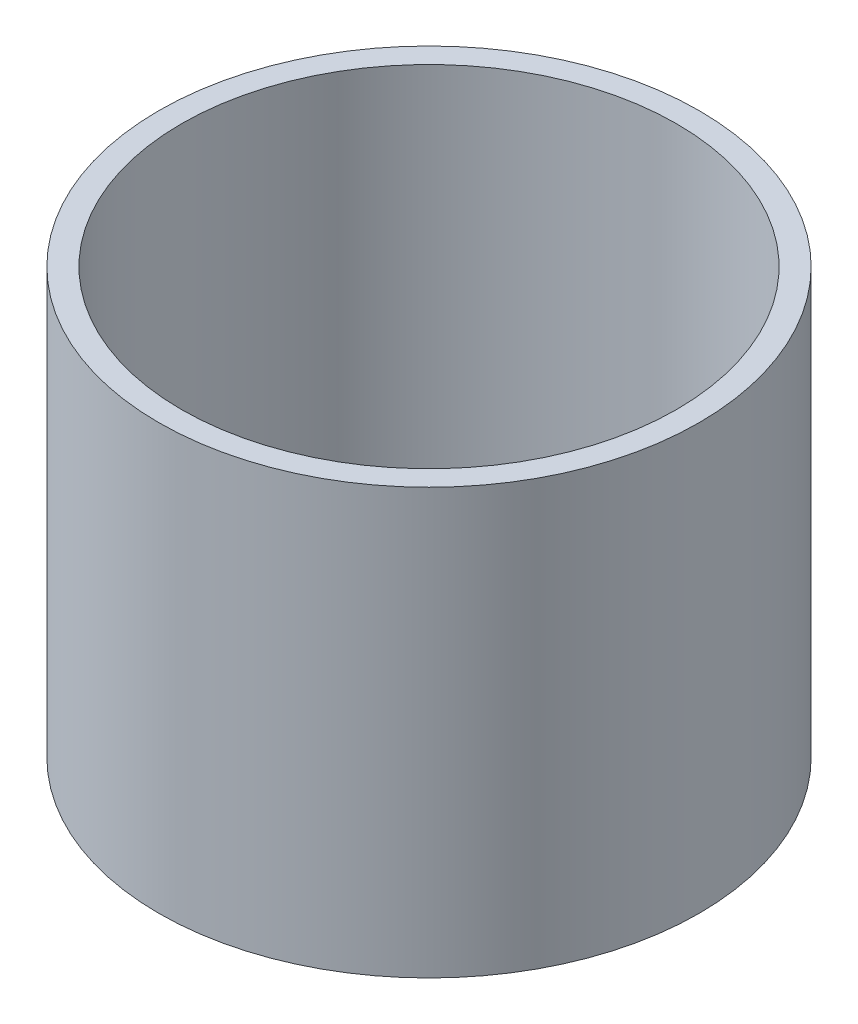
SolidWorks part; units mm, degrees
material "STK400"
ref_plane "Front Plane" through (0, 0, 0) normal (0, 0, 1) x (1, 0, 0)
ref_plane "Top Plane" through (0, 0, 0) normal (0, 1, 0) x (1, 0, 0)
ref_plane "Right Plane" through (0, 0, 0) normal (1, 0, 0) x (0, 0, -1)
sketch "Sketch1" plane through (0, 0, 0) normal (0, 1, 0) x (1, 0, 0)
  circle A0 centre (0, 0) radius 38.15
  circle A1 centre (0, 0) radius 34.95
  dimension "D1" = 76.3
  dimension "D2" = 3.2
extrude "Boss-Extrude1" add sketch "Sketch1" along normal blind 60
